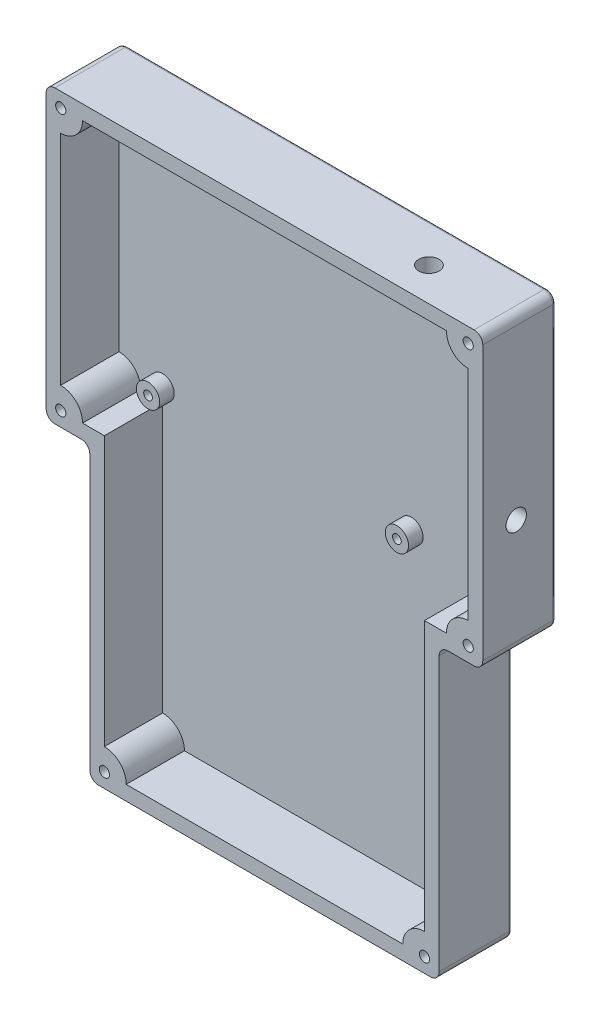
from build123d import *

# Parameters (mm, degrees)
BOSS_EXTRUDE1_DEPTH = 25
CUT_EXTRUDE1_DEPTH  = 20
FILLET1_R           = 3
FILLET2_R           = 1
SKETCH5_R           = 4
SKETCH5_R_2         = 1.5
BOSS_EXTRUDE2_DEPTH = 5
BOSS_EXTRUDE3_DEPTH = 25
SKETCH7_R           = 1.75
CUT_EXTRUDE4_DEPTH  = 20
SKETCH8_R           = 3.75
CUT_EXTRUDE5_DEPTH  = 8
CUT_EXTRUDE6_REACH  = 253.247
SKETCH9_R           = 3.5
CUT_EXTRUDE7_REACH  = 217.058
SKETCH10_R          = 3.5


with BuildPart() as part:
    # Sketch1 → Boss-Extrude1 (new body)
    with BuildSketch(Plane.XY):
        Polygon((75, 200), (-75, 200), (-75, 100), (-60, 100), (-60, 0), (60, 0), (60, 100), (75, 100), align=None)
    extrude(amount=BOSS_EXTRUDE1_DEPTH)

    # Sketch2 → Cut-Extrude1 (cut)
    with BuildSketch(Plane.XY.offset(25)):
        Polygon((70, 105), (70, 195), (-70, 195), (-70, 105), (-55, 105), (-55, 5), (55, 5), (55, 105), align=None)
    extrude(amount=-CUT_EXTRUDE1_DEPTH, mode=Mode.SUBTRACT)

    # Fillet1
    fillet1_edges = [part.edges().sort_by_distance(p)[0] for p in [
        (-75, 100, 12.5),
        (-75, 200, 12.5),
        (75, 200, 12.5),
        (75, 100, 12.5),
        (60, 100, 12.5),
        (60, 0, 12.5),
        (-60, 0, 12.5),
        (-60, 100, 12.5),
    ]]
    fillet(fillet1_edges, radius=FILLET1_R)

    # Fillet2
    fillet2_edges = [part.edges().sort_by_distance(p)[0] for p in [
        (67.5, 100, 0),
        (60, 50, 0),
        (-60, 50, 0),
        (-67.5, 100, 0),
        (0, 0, 0),
        (-75, 150, 0),
        (0, 200, 0),
        (75, 150, 0),
        (-74.121320344, 199.121320344, 0),
        (-74.121320344, 100.878679656, 0),
        (74.121320344, 199.121320344, 0),
        (74.121320344, 100.878679656, 0),
        (59.121320344, 0.878679656, 0),
        (-59.121320344, 0.878679656, 0),
        (60.878679656, 99.121320344, 0),
        (-60.878679656, 99.121320344, 0),
    ]]
    fillet(fillet2_edges, radius=FILLET2_R)

    # Sketch5 → Boss-Extrude2 (add)
    # profile 1 of 4: a face of its own
    with BuildSketch(Plane.XY.offset(5)):
        with Locations((-55, 190.5)):
            Circle(SKETCH5_R)
        with Locations((-55, 190.5)):
            Circle(SKETCH5_R_2, mode=Mode.SUBTRACT)
    # profile 2 of 4: a face of its own
    with BuildSketch(Plane.XY.offset(5)):
        with Locations((30.5, 190.5)):
            Circle(SKETCH5_R)
        with Locations((30.5, 190.5)):
            Circle(SKETCH5_R_2, mode=Mode.SUBTRACT)
    # profile 3 of 4: a face of its own
    with BuildSketch(Plane.XY.offset(5)):
        with Locations((-55, 109.5)):
            Circle(SKETCH5_R)
        with Locations((-55, 109.5)):
            Circle(SKETCH5_R_2, mode=Mode.SUBTRACT)
    # profile 4 of 4: a face of its own
    with BuildSketch(Plane.XY.offset(5)):
        with Locations((30.5, 109.5)):
            Circle(SKETCH5_R)
        with Locations((30.5, 109.5)):
            Circle(SKETCH5_R_2, mode=Mode.SUBTRACT)
    extrude(amount=BOSS_EXTRUDE2_DEPTH)

    # Sketch6 → Boss-Extrude3 (add)
    with BuildSketch(Plane.XY.offset(25)):
        with BuildLine():
            Line((-71.747064875, 196.748861378), (-62.706750801, 196.748861378))
            ThreePointArc((-62.706750801, 196.748861378), (-64.696046035, 189.697352328), (-71.747064875, 187.706320248))
            Line((-71.747064875, 187.706320248), (-71.747064875, 196.748861378))
        make_face()
        with BuildLine():
            Line((71.50031539, 195.771596957), (62.539796374, 195.771596957))
            ThreePointArc((62.539796374, 195.771596957), (64.963763881, 189.442453262), (71.50031539, 187.651595157))
            Line((71.50031539, 187.651595157), (71.50031539, 195.771596957))
        make_face()
        with BuildLine():
            Line((71.50031539, 103.139966112), (62.734308434, 103.139966112))
            ThreePointArc((62.734308434, 103.139966112), (64.567806467, 110.171196518), (71.50031539, 112.348404843))
            Line((71.50031539, 112.348404843), (71.50031539, 103.139966112))
        make_face()
        with BuildLine():
            Line((-56.424780788, 4.339960717), (-47.529099911, 4.339960717))
            ThreePointArc((-47.529099911, 4.339960717), (-49.976766301, 10.56930186), (-56.424780788, 12.363423097))
            Line((-56.424780788, 12.363423097), (-56.424780788, 4.339960717))
        make_face()
        with BuildLine():
            Line((56.315887188, 4.339960717), (47.529099911, 4.339960717))
            ThreePointArc((47.529099911, 4.339960717), (49.935780208, 10.532059101), (56.315887188, 12.3836604))
            Line((56.315887188, 12.3836604), (56.315887188, 4.339960717))
        make_face()
        with BuildLine():
            Line((-71.747064875, 102.631768342), (-62.883717346, 102.631768342))
            ThreePointArc((-62.883717346, 102.631768342), (-64.473223551, 110.069984427), (-71.747064875, 112.293679752))
            Line((-71.747064875, 112.293679752), (-71.747064875, 102.631768342))
        make_face()
    extrude(amount=-BOSS_EXTRUDE3_DEPTH)

    # Sketch7 → Cut-Extrude4 (cut)
    with BuildSketch(Plane.XY.offset(25)):
        with Locations((-70, 195)):
            Circle(SKETCH7_R)
        with Locations((-70, 105)):
            Circle(SKETCH7_R)
        with Locations((-55, 5)):
            Circle(SKETCH7_R)
        with Locations(Location((55, 5, 0), (0, 0, 180))):
            Circle(SKETCH7_R)
        with Locations(Location((70, 105, 0), (0, 0, 180))):
            Circle(SKETCH7_R)
        with Locations(Location((70, 195, 0), (0, 0, 180))):
            Circle(SKETCH7_R)
    extrude(amount=-CUT_EXTRUDE4_DEPTH, mode=Mode.SUBTRACT)

    # Sketch8 → Cut-Extrude5 (cut)
    with BuildSketch(Plane(origin=(0, 0, 0), x_dir=(-1, 0, 0), z_dir=(0, 0, -1))):
        with Locations((-70, 195)):
            Circle(SKETCH8_R)
        with Locations((-70, 105)):
            Circle(SKETCH8_R)
        with Locations((-55, 5)):
            Circle(SKETCH8_R)
        with Locations(Location((55, 5, 0), (0, 0, 180))):
            Circle(SKETCH8_R)
        with Locations(Location((70, 105, 0), (0, 0, 180))):
            Circle(SKETCH8_R)
        with Locations(Location((70, 195, 0), (0, 0, 180))):
            Circle(SKETCH8_R)
    extrude(amount=-CUT_EXTRUDE5_DEPTH, mode=Mode.SUBTRACT)

    # Sketch9 → Cut-Extrude6 (cut, up to next)
    with BuildSketch(Plane(origin=(75, 0, 0), x_dir=(0, 0, -1), z_dir=(1, 0, 0)), mode=Mode.PRIVATE) as cut_extrude6_sk1:
        with Locations(Location((-13.5, 139.14, 0), (0, 0, 90))):
            Circle(SKETCH9_R)
    cut_extrude6_tool1 = extrude(cut_extrude6_sk1.sketch, amount=-CUT_EXTRUDE6_REACH, mode=Mode.PRIVATE) & part.part
    add(cut_extrude6_tool1.solids().sort_by_distance((75, 139.14, 13.5))[0], mode=Mode.SUBTRACT)

    # Sketch10 → Cut-Extrude7 (cut, up to next)
    with BuildSketch(Plane(origin=(0, 200, 0), x_dir=(1, 0, 0), z_dir=(0, 1, 0)), mode=Mode.PRIVATE) as cut_extrude7_sk1:
        with Locations(Location((45, -13.5, 0), (0, 0, 270))):
            Circle(SKETCH10_R)
    cut_extrude7_tool1 = extrude(cut_extrude7_sk1.sketch, amount=-CUT_EXTRUDE7_REACH, mode=Mode.PRIVATE) & part.part
    add(cut_extrude7_tool1.solids().sort_by_distance((45, 200, 13.5))[0], mode=Mode.SUBTRACT)


solid = part.part
